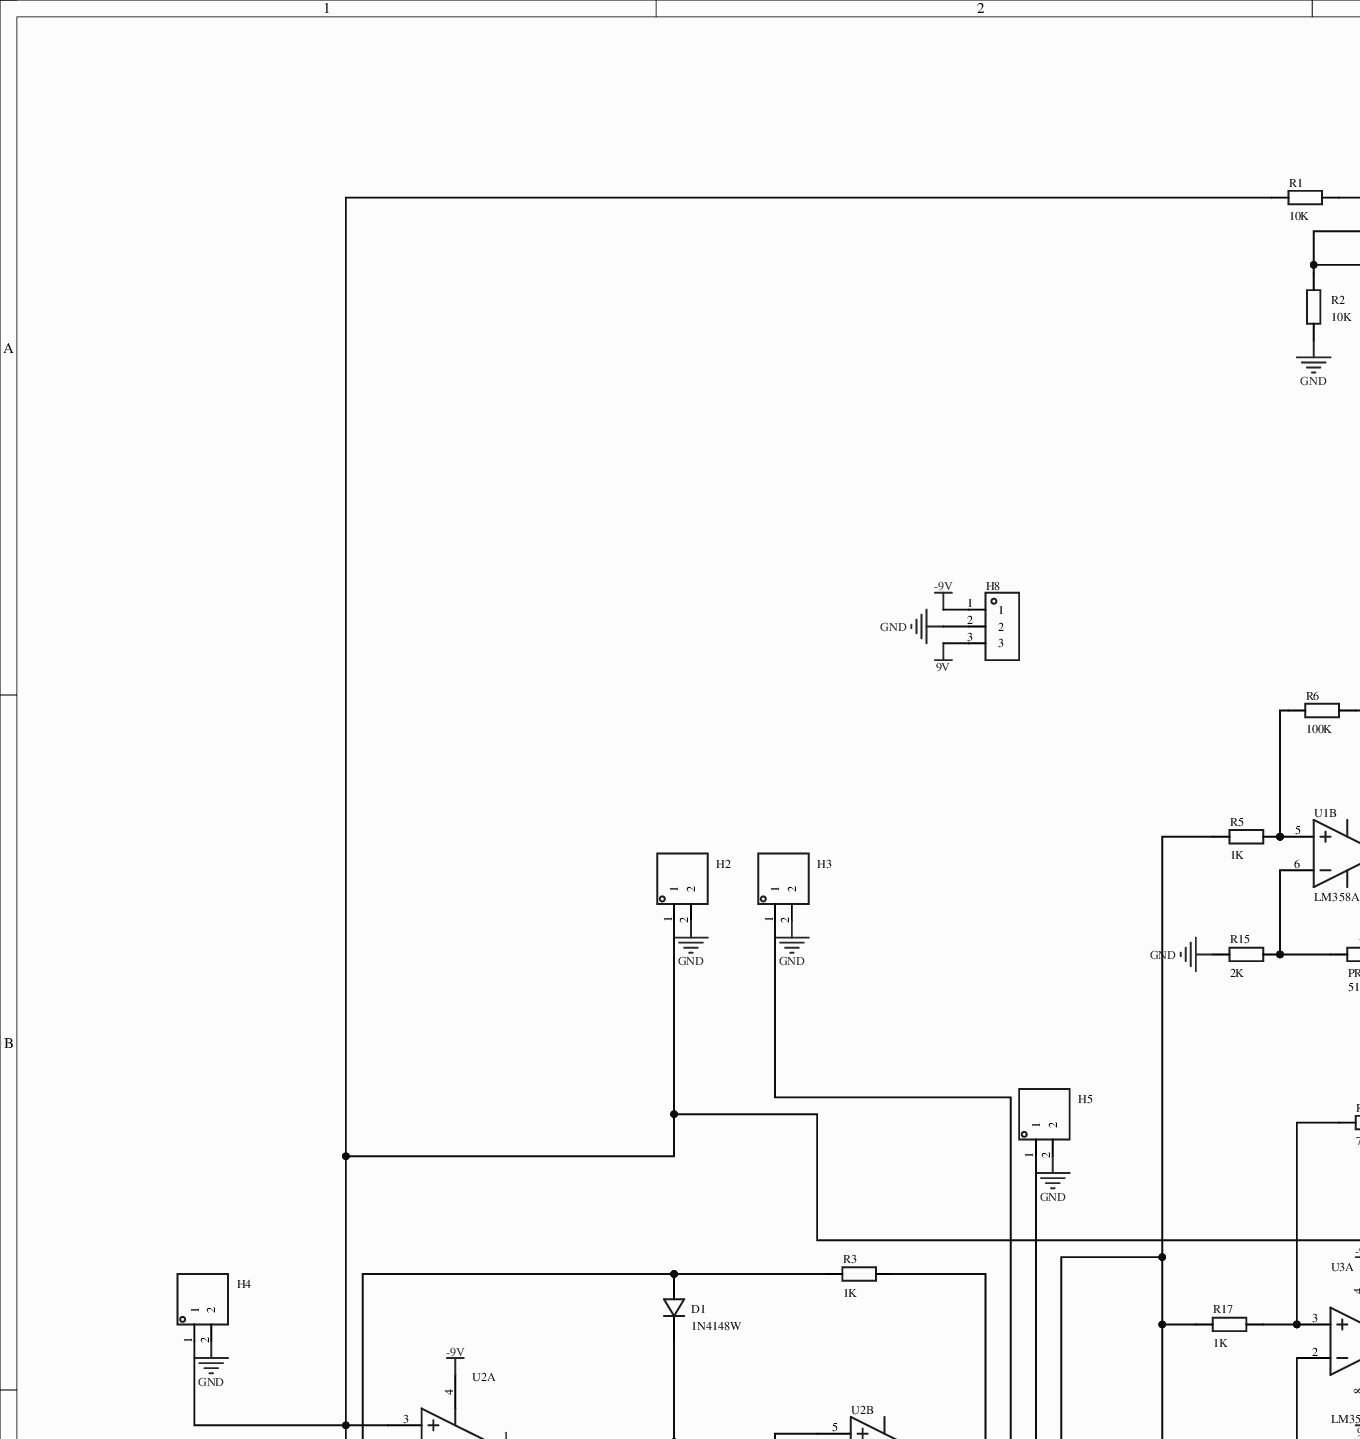
[diagram p0: MISC51795-3.schdoc, top left]
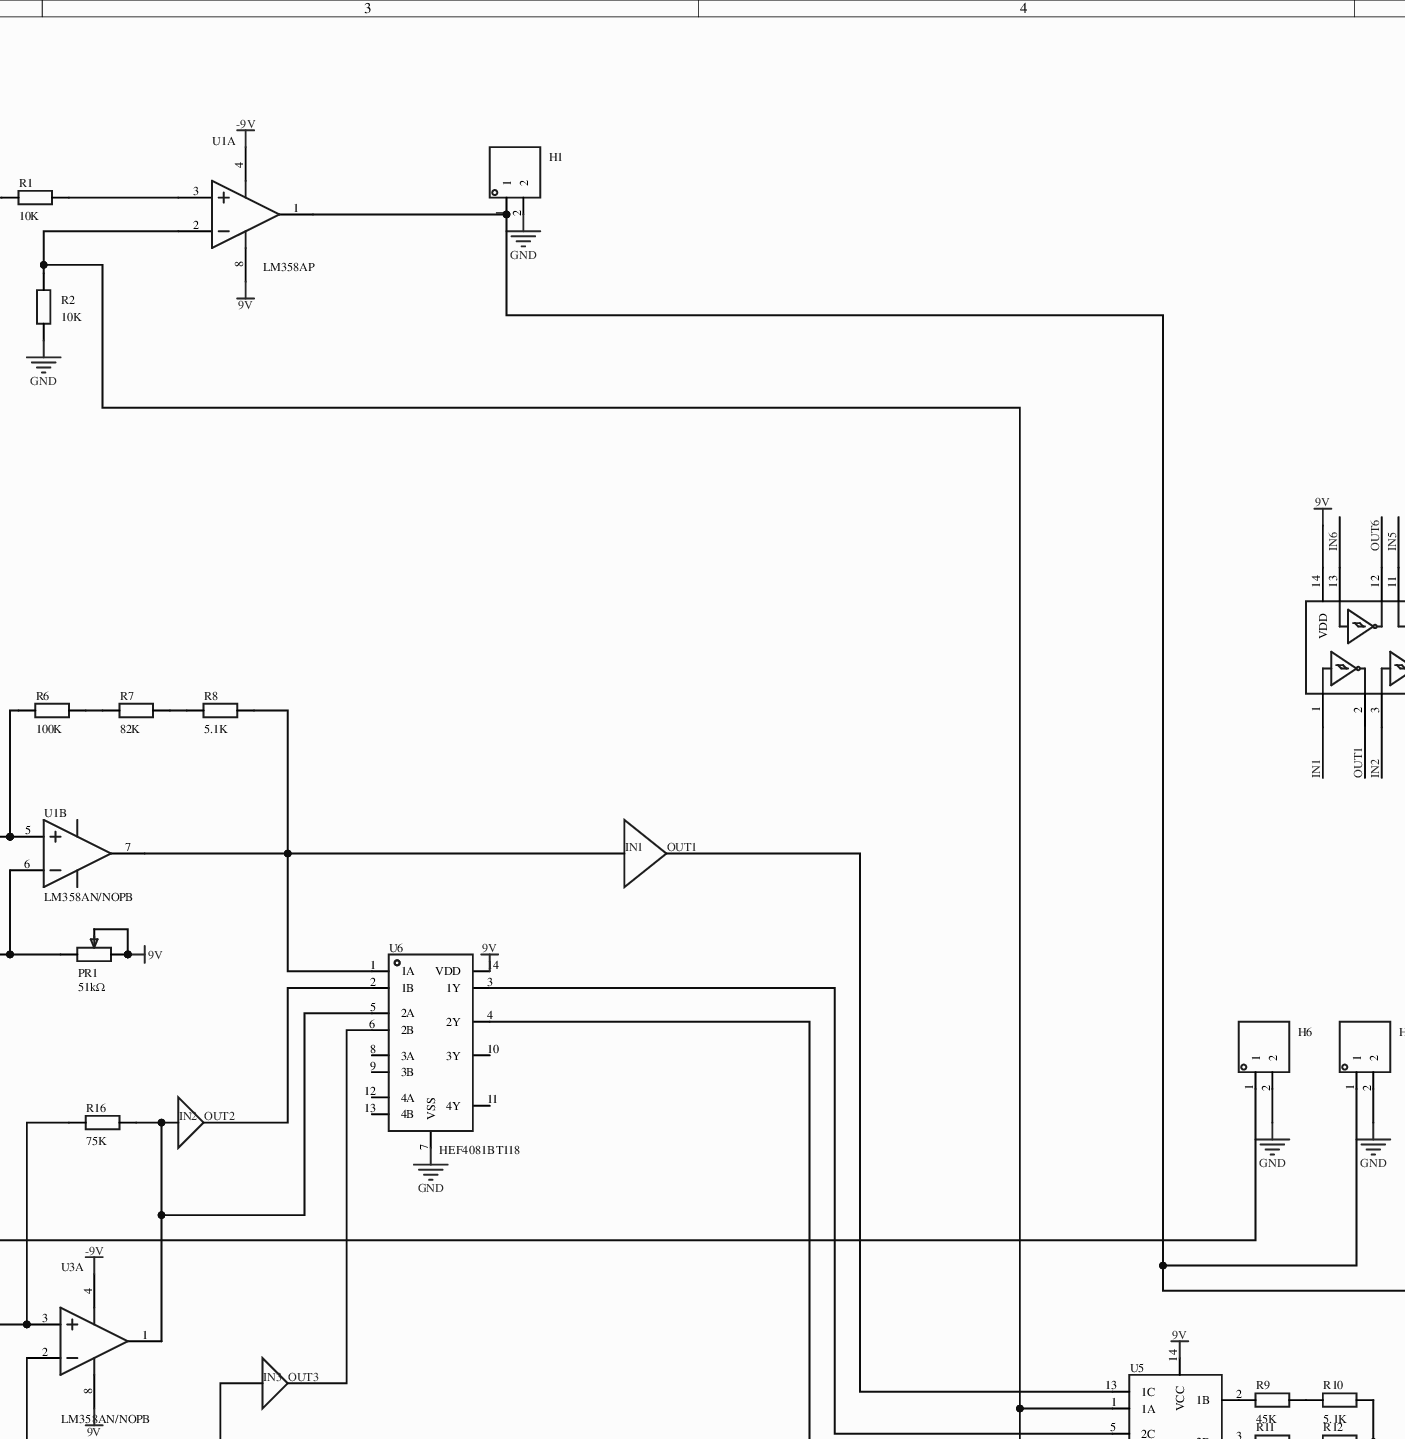
[diagram p1: MISC51795-3.schdoc, top middle]
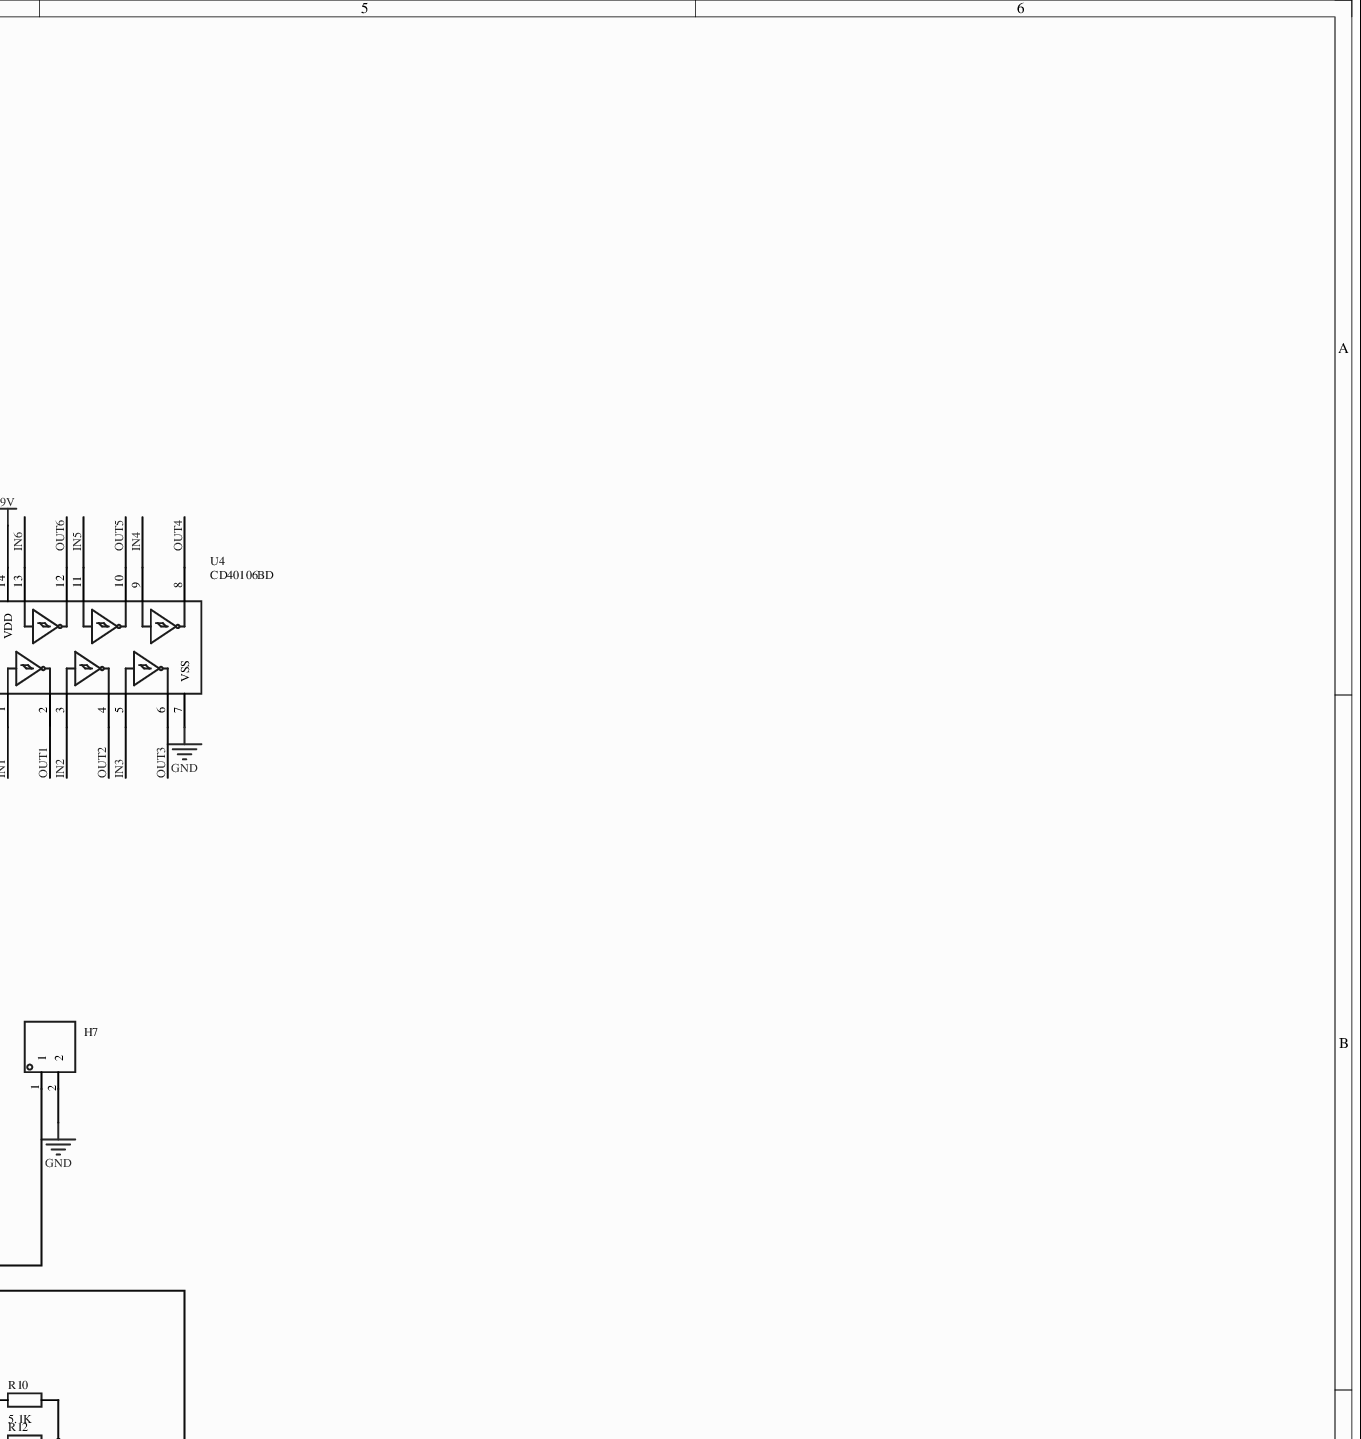
[diagram p2: MISC51795-3.schdoc, top right]
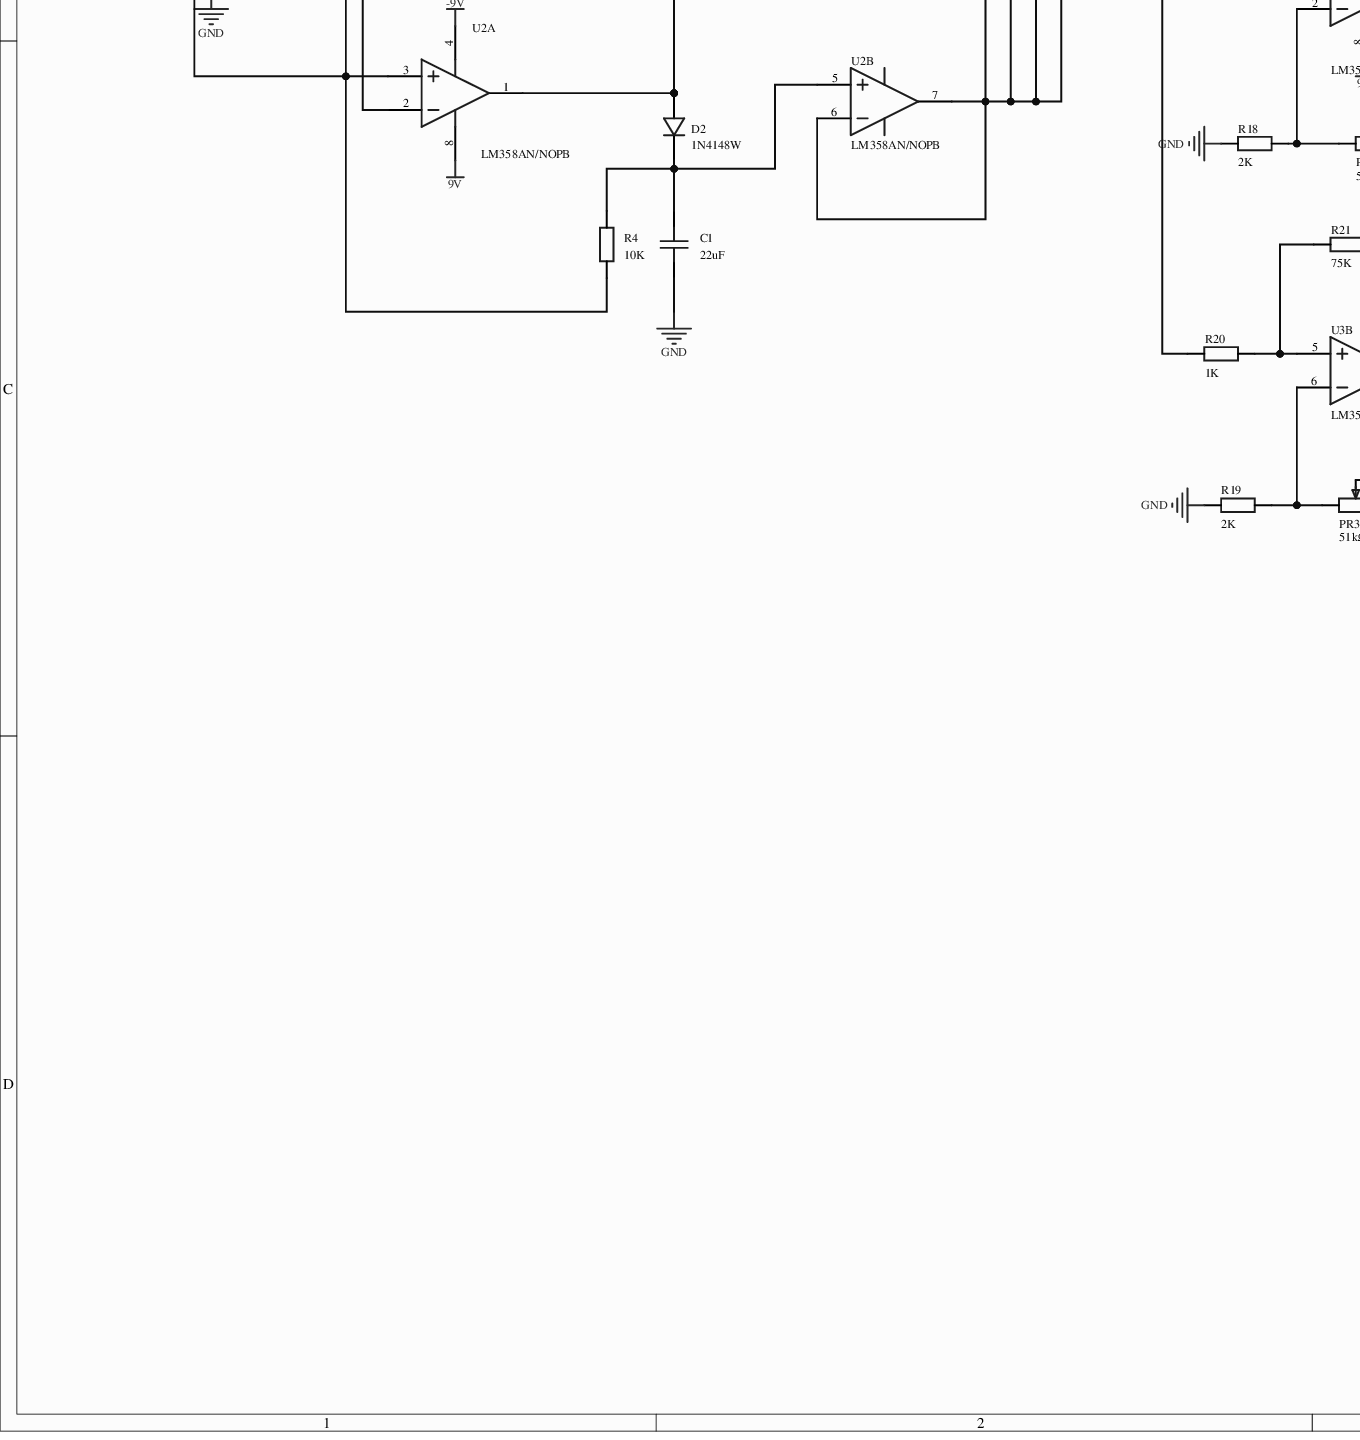
[diagram p3: MISC51795-3.schdoc, bottom left]
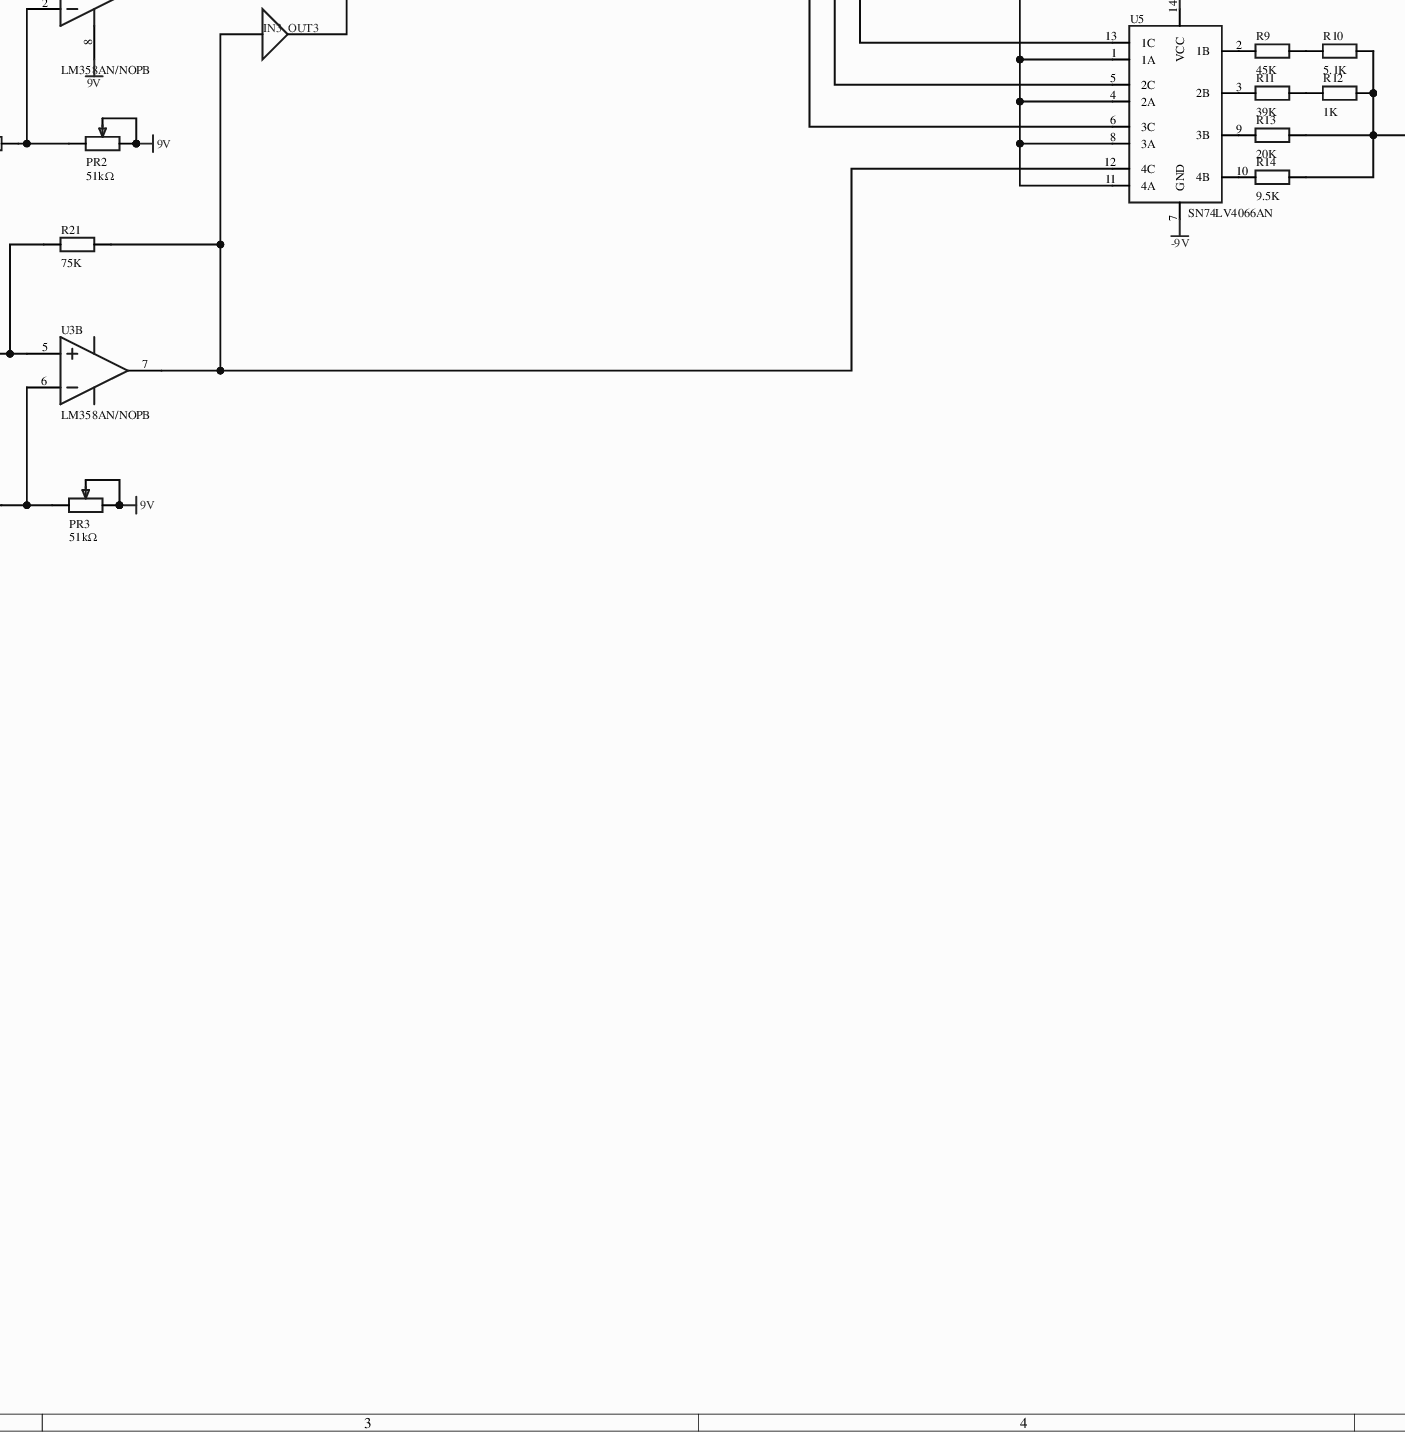
[diagram p4: MISC51795-3.schdoc, bottom middle]
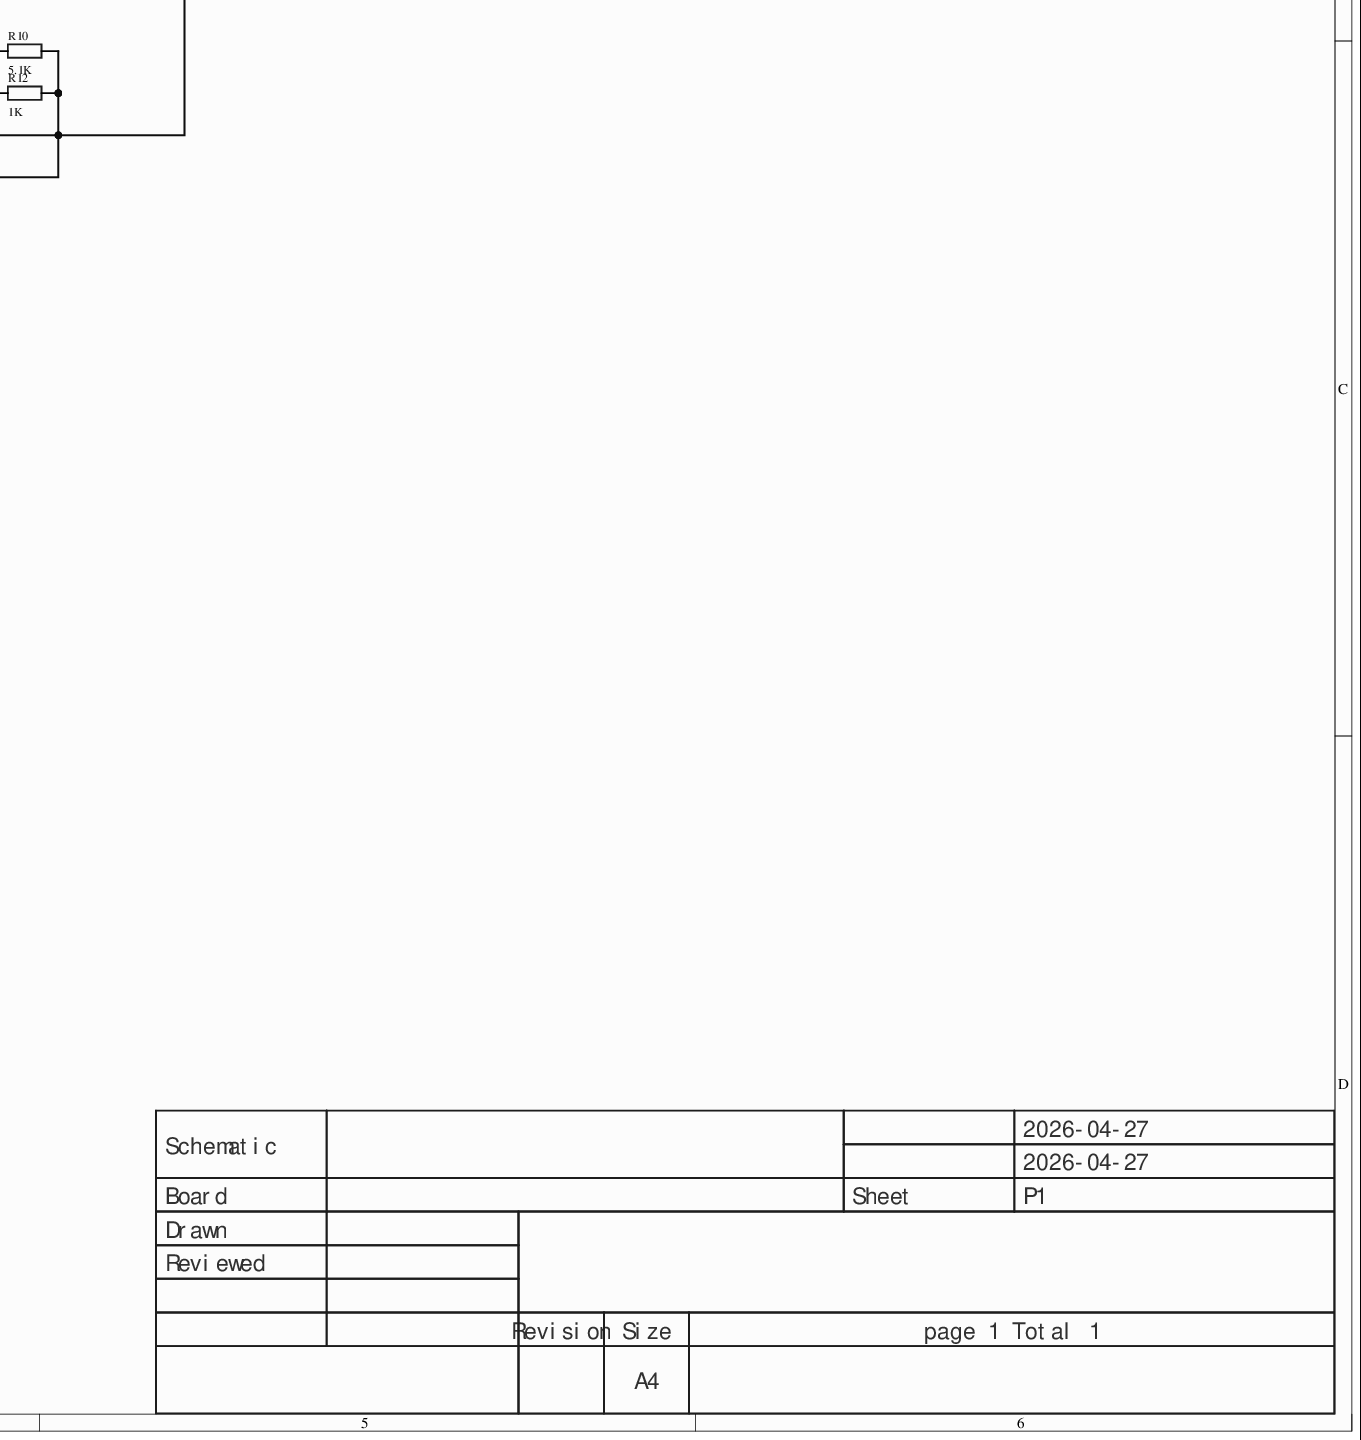
[diagram p5: MISC51795-3.schdoc, bottom right]
# Altium project MISC51795-2.PrjPcb
1 sheet, 41 parts. Net scope: global (net labels, ports and power ports of the same name join across sheets).
Board file: MISC51795.pcbdoc

## Sheet MISC51795-3.schdoc
size 594 x 419 mm; Version: V1.0; @Project Name: MISC51795; @Update Date: 2026-04-27; @Create Date: 2026-04-27; @Board Name: MISC51795; @Create Time: 12:42:14; @Page Count: 1; @Page No: 1; @Schematic Name: MISC51795; @Update Time: 12:42:14; Size: A4

### Parts
C1  22uF  [CAP-TH_L5.0-W2.5-P5.00-D1.0]
D1  1N4148W  [SOD-123F_L2.7-W1.6-LS3.8-RD]
D2  1N4148W  [SOD-123F_L2.7-W1.6-LS3.8-RD]
H1  (no value)  [HDR-TH_2P-P2.54-V-M-1]
H2  (no value)  [HDR-TH_2P-P2.54-V-M-1]
H3  (no value)  [HDR-TH_2P-P2.54-V-M-1]
H4  (no value)  [HDR-TH_2P-P2.54-V-M-1]
H5  (no value)  [HDR-TH_2P-P2.54-V-M-1]
H6  (no value)  [HDR-TH_2P-P2.54-V-M-1]
H7  (no value)  [HDR-TH_2P-P2.54-V-M-1]
H8  (no value)  [HDR-TH_3P-P2.54-V-F]
PR1  51kΩ  [R_3296]
PR2  51kΩ  [R_3296]
PR3  51kΩ  [R_3296]
R1  10K  [Res_1/8W]
R2  10K  [Res_1/8W]
R3  1K  [Res_1/8W]
R4  10K  [Res_1/8W]
R5  1K  [Res_1/8W]
R6  100K  [Res_1/8W]
R7  82K  [Res_1/8W]
R8  5.1K  [Res_1/8W]
R9  45K  [Res_1/8W]
R10  5.1K  [Res_1/8W]
R11  39K  [Res_1/8W]
R12  1K  [Res_1/8W]
R13  20K  [Res_1/8W]
R14  9.5K  [Res_1/8W]
R15  2K  [Res_1/8W]
R16  75K  [Res_1/8W]
R17  1K  [Res_1/8W]
R18  2K  [Res_1/8W]
R19  2K  [Res_1/8W]
R20  1K  [Res_1/8W]
R21  75K  [Res_1/8W]
U1  LM358AP  [PDIP-8_L10.2-W6.5-P2.54-LS7.6-BL]  (parts A,B of 2)
U2  LM358AN/NOPB  [PDIP-8_L10.2-W6.5-P2.54-LS7.6-BL]  (parts A,B of 2)
U3  LM358AN/NOPB  [PDIP-8_L10.2-W6.5-P2.54-LS7.6-BL]  (parts A,B of 2)
U4  CD40106BD  [DIP-14_L19.1-W6.4-P2.54-LS7.6-BL]
U5  SN74LV4066AN  [PDIP-14_L19.3-W6.4-P2.54-LS7.9-BL-1]
U6  HEF4081BT118  [SO-14_L8.9-W3.9-P1.27-LS6.0-BL]

### Nets
9V: H8.3 PR1.1 PR1.2 PR2.1 PR2.2 PR3.1 PR3.2 U1.8(V+) U2.8(V+) U3.8(V+) U4.14(VDD) U5.14(VCC) U6.14(VDD)
-9V: H8.1 U1.4(GND) U2.4(GND) U3.4(GND) U5.7(GND)
GND: C1.1 H1.2 H2.2 H3.2 H4.2 H5.2 H6.2 H7.2 H8.2 R2.1 R15.1 R18.1 R19.1 U4.7(VSS) U6.7(VSS)
IN1: R8.2 U1.7(OUTB) U4.1 U6.1(1A)
IN2: R16.2 U3.1(OUTA) U4.3 U6.5(2A)
IN3: R21.2 U3.7(OUTB) U4.5 U5.12(4C)
IN4: U4.9
IN5: U4.11
IN6: U4.13
OUT1: U4.2 U5.13(1C)
OUT2: U4.4 U6.2(1B)
OUT3: U4.6 U6.6(2B)
OUT4: U4.8
OUT5: U4.10
OUT6: U4.12
NetC1_2: C1.2 D2.1(K) R4.2 U2.5(INB+)
NetD1_1: D1.1(K) D2.2(A) U2.1(OUTA)
NetD1_2: D1.2(A) R3.1 U2.2(INA-)
NetH1_1: H1.1 H7.1 R10.2 R12.2 R13.2 R14.2 U1.1(OUTA)
NetH2_1: H2.1 H4.1 H6.1 R1.1 R4.1 U2.3(INA+)
NetH3_1: H3.1 H5.1 R3.2 R5.1 R17.1 R20.1 U2.6(INB-) U2.7(OUTB)
NetPR1_3: PR1.3 R15.2 U1.6(INB-)
NetPR2_3: PR2.3 R18.2 U3.2(INA-)
NetPR3_3: PR3.3 R19.2 U3.6(INB-)
NetR1_2: R1.2 U1.3(INA+)
NetR2_2: R2.2 U1.2(INA-) U5.1(1A) U5.4(2A) U5.8(3A) U5.11(4A)
NetR5_2: R5.2 R6.1 U1.5(INB+)
NetR6_2: R6.2 R7.1
NetR7_2: R7.2 R8.1
NetR9_1: R9.1 U5.2(1B)
NetR9_2: R9.2 R10.1
NetR11_1: R11.1 U5.3(2B)
NetR11_2: R11.2 R12.1
NetR13_1: R13.1 U5.9(3B)
NetR14_1: R14.1 U5.10(4B)
NetR16_1: R16.1 R17.2 U3.3(INA+)
NetR20_2: R20.2 R21.1 U3.5(INB+)
NetU5_5: U5.5(2C) U6.3(1Y)
NetU5_6: U5.6(3C) U6.4(2Y)

Not connected (* = marked no-connect by the designer): U6 8(3A) 9(3B) 10(3Y) 11(4Y) 12(4A) 13(4B)

### Notes on the sheet
- 2026-04-27
- Schematic
- Board
- Sheet
- P1
- Drawn
- Reviewed
- Revision
- Size
- A4
- page 1 Total 1

### Library data of the parts
C1 = CAP_0603: Symbol: Capacitance; ConvertToPcb: yes; ModelId: ac125912035d415993ca9572d50418b10819f05c4eef4c71ace90d822a990e87; ModelName: C0603_L1.6-W0.8-H0.8; ModelTransform: 62.992,31.496,0,0,0,0,0,0,0; Device: CAP_0603; Value: 22uF; AddInBom: yes; Supplier Footprint: 0603; FootprintName: CAP-TH_L5.0-W2.5-P5.00-D1.0
D1 D2 = 1N4148W_C81598: Diode configuration: independent; forward voltage (Vf): 1V@50mA; DC reverse voltage (Vr): 75V; rectified current: 150mA; reverse recovery time (Trr): 4ns;; Manufacturer: ST(先科); AddInBom: yes; ModelId: 7091c985327f41e7b1e4fbd3002f031e0819f05c4eef4c71ace90d822a990e87; ModelTransform: 149.606,62.992,0,0,0,0,0,0,0; Pd - Power Dissipation: 400mW; Reverse Leakage Current (Ir): 1uA@75V; Non-Repetitive Peak Forward Surge Current: 1A; Symbol: 1N4148W_C81598; Device: 1N4148W_C81598; LCSC Part Name: 1N4148W; SupplierPart: C81598; ManufacturerPart: 1N4148W; Supplier Footprint: SOD-123; JLCPCB Part Class: Basic Part; Datasheet: https://example.com/datasheet/1N4148W/82750.html; Supplier: LCSC; ConvertToPcb: yes; FootprintName: SOD-123F_L2.7-W1.6-LS3.8-RD; ModelName: SOD-123F_L2.7-W1.6-LS3.8-RD; Diode Configuration: Independent; Voltage - Forward(Vf@If): 1V@50mA; Voltage - DC Reverse(Vr): 75V; Current - Rectified: 150mA; Reverse Recovery Time (trr): 4ns; Operating Junction Temperature Range: -
H1-H7 = HDR-M_2.54_1x2P: Symbol: 210S-1*2P L=11.6MMGold-plated black; ConvertToPcb: yes; ModelId: 79b2e9f2d70a4d68a1b7098f27c6d4c50819f05c4eef4c71ace90d822a990e87; ModelName: HDR-M-2.54_1x2; ModelTransform: 200,100,0,0,0,0,0,0,-118.11; Device: HDR-M_2.54_1x2P; AddInBom: yes; SupplierPart: C124375; Supplier Footprint: 插件; FootprintName: HDR-TH_2P-P2.54-V-M-1
H8 = HDR-F_2.54_1x3P: Symbol: PM254V-11-03-H85; ConvertToPcb: yes; ModelId: f3b3cc5aae9641bf9e56fc160cef875b0819f05c4eef4c71ace90d822a990e87; ModelName: HDR2.54-F-LI-1X3P; ModelTransform: 299.9994,100,0,0,0,0,0,0,-118.11; Device: HDR-F_2.54_1x3P; AddInBom: yes; SupplierPart: C541850; Supplier Footprint: 插件; FootprintName: HDR-TH_3P-P2.54-V-F
PR1-PR3 = R_3296: ConvertToPcb: yes; ModelId: b182808559bb43bda9e7de64b64134cb0819f05c4eef4c71ace90d822a990e87; ModelName: 3296W; ModelTransform: 373.98,188.96,590.49,180,0,0,0,0,-140; Symbol: R_3296; Device: R_3296; Value: 51kΩ; AddInBom: yes; Supplier Footprint: 直插; FootprintName: R_3296
R1-R21 = Res_0603: Symbol: Resistor; ConvertToPcb: yes; ModelId: fc143cca1e79419f9cd78b61e9279f080819f05c4eef4c71ace90d822a990e87; ModelName: R0603; ModelTransform: 31.8897,63.7794,0,90,0,0,0,0,0; Device: Res_0603; AddInBom: yes; Supplier Footprint: 0603; FootprintName: Res_1/8W
  R1 R2 R4: Value: 10K
  R3 R5 R12 R17 R20: Value: 1K
  R6: Value: 100K
  R7: Value: 82K
  R8 R10: Value: 5.1K
  R9: Value: 45K
  R11: Value: 39K
  R13: Value: 20K
  R14: Value: 9.5K
  R15 R18 R19: Value: 2K
  R16 R21: Value: 75K
U1-U3 = LM358AN/NOPB: Amplifiers: 2; rail-to-rail: -; GBW: 1MHz; input offset voltage (Vos): 2mV; slew rate (SR): -; input bias current (Ib): 50nA;; Manufacturer: TI(德州仪器); Relevance: []; AddInBom: yes; ModelId: b5bb019b7dad497cba3f645155e53c260819f05c4eef4c71ace90d822a990e87; ModelTransform: 401.574,311.8104,0,0,0,0,0,0,-137.795; Number of Channels: 2; Maximum Power Supply Range (Vdd-Vss): 32V; Input Offset Voltage Drift(Vos TC): 7uV/℃; Common Mode Rejection Ratio(CMRR): 85dB; Quiescent Current: 500uA; Output Current: 40mA; Single supply: 3V~32V; Dual Supply: -16V~-1.5V; 1.5V~16V; Symbol: LM358AN/NOPB; Device: LM358AN/NOPB; LCSC Part Name: LM358AN/NOPB; SupplierPart: C1348620; Supplier Footprint: PDIP-8; JLCPCB Part Class: Extended Part; Supplier: LCSC; ConvertToPcb: yes; FootprintName: PDIP-8_L10.2-W6.5-P2.54-LS7.6-BL; ModelName: PDIP-8_L10.2-W6.5-P2.54-LS7.6-BL; Rail to Rail: -; Gain Bandwidth Product: 1MHz; Vos - Input Offset Voltage: 2mV; Slew Rate: -; Ib - Input Bias Current: 50nA; Input Offset Current(Ios): 50nA; Input Voltage Noise Density: -; Input offset current drift(Ios TC): -; Operating Temperature: 0℃~+70℃
  U1: Manufacturer Part: LM358AP
  U2 U3: ManufacturerPart: LM358AN/NOPB
U4 = CD40106BD: Input type: Schmitt trigger; operating voltage: 3V~15V; quiescent current (Iq): 16uA; channels: 6; propagation delay (tpd): 80ns@10V, 50pF; 70ns@15V, 50pF; 220ns@5V, 50pF;; Manufacturer: Sungine(双竞集成); AddInBom: yes; ModelId: 4fb82330961949e587245d1f3ebad69c0819f05c4eef4c71ace90d822a990e87; ModelTransform: 751.967,324.8025,0,0,0,0,0,0,-118.11; Number of Circuits: 6; Number of Inputs: 1; Output Logic Level - High: 9.95V; 4.95V; 14.95V; Output Logic Level - Low: 50mV; Symbol: CD40106BD; Device: CD40106BD; LCSC Part Name: 六CMOS施密特触发器; SupplierPart: C5274709; ManufacturerPart: CD40106BD; Supplier Footprint: DIP-14; JLCPCB Part Class: Extended Part; Datasheet: https://example.com/datasheet/CD40106BD/6005847.html; Supplier: LCSC; ConvertToPcb: yes; FootprintName: DIP-14_L19.1-W6.4-P2.54-LS7.6-BL; ModelName: DIP-14_L19.1-W6.4-P2.54-LS7.6-BL; Input Type: Schmitt trigger; Voltage - Supply: 3V~15V; Quiescent Current(Iq): 16uA; Current - Output Low(IOL): -; Current - Output High(IOH): -; Input Logic Level - High: -; Input Logic Level -Low: -; Propagation Delay: 80ns@10V, 50pF; 70ns@15V, 50pF; 220ns@5V, 50pF; Series: -; Operating Temperature: -10℃~+70℃
U5 = SN74LV4066AN: Switch circuit: SPST-NO; channels: 4; on-resistance (Ron@VCC): 75Ω;; Manufacturer: TI(德州仪器); Symbol: SN74LV4066AN_1; AddInBom: yes; ModelId: 850da569defe42bfb44bffbf615858220819f05c4eef4c71ace90d822a990e87; ModelTransform: 751.967,309.842,0,0,0,0,0,0,-118.11; Number of Channels: 4; Supply Voltage: 2V~5.5V; Turn-on time: 12ns; Device: SN74LV4066AN; LCSC Part Name: SN74LV4066AN; SupplierPart: C1546548; ManufacturerPart: SN74LV4066AN; Supplier Footprint: PDIP-14; JLCPCB Part Class: Extended Part; Supplier: LCSC; ConvertToPcb: yes; FootprintName: PDIP-14_L19.3-W6.4-P2.54-LS7.9-BL-1; ModelName: PDIP-14_L19.3-W6.4-P2.54-LS7.9-BL-1; Switch Circuit: SPST-NO; On-State Resistance (Max): 75Ω; Turn-off time: 12ns
U6 = HEF4081BT118: Logic type: AND gate; channels: 4; operating voltage: 3V~15V; quiescent current (Iq): 1uA; propagation delay (tpd): 50ns@10V, 50pF; 110ns@5V, 50pF; 40ns@15V, 50pF;; Manufacturer: Nexperia(安世); AddInBom: yes; ModelId: b93533fd67a84aecab96c4d693158bad0819f05c4eef4c71ace90d822a990e87; ModelName: SO-14_L8.9-W3.9-H1.5-P1.27-LS6.0-BL; ModelTransform: 350.393,236.22,0,0,0,0,-0.0005,0,0; Number of Channels: 4; Current - Output Low(IOL): 4.2mA; Input Logic Level - High: 11V; 7V; 3.5V; Input Logic Level - Low: 1.5V; 3V; 4V; Output Logic Level - High: 14.95V; 9.95V; 4.95V; Output Logic Level - Low: 50mV; Input Number: 2; Symbol: HEF4081BT118; Device: HEF4081BT118; LCSC Part Name: HEF4081BT118; SupplierPart: C4472069; ManufacturerPart: HEF4081BT118; Supplier Footprint: SO-14; JLCPCB Part Class: Extended Part; Datasheet: https://example.com/datasheet/HEF4081BT118/5043137.html; Supplier: LCSC; ConvertToPcb: yes; FootprintName: SO-14_L8.9-W3.9-P1.27-LS6.0-BL; Logic Type: AND gate; Voltage - Supply: 3V~15V; Quiescent Current: 1uA; Current - Output High(IOH): 4.2mA; Series: HEF4081B; Propagation Delay: 50ns@10V, 50pF; 110ns@5V, 50pF; 40ns@15V, 50pF; Operating Temperature: -40℃~+125℃; Features: -